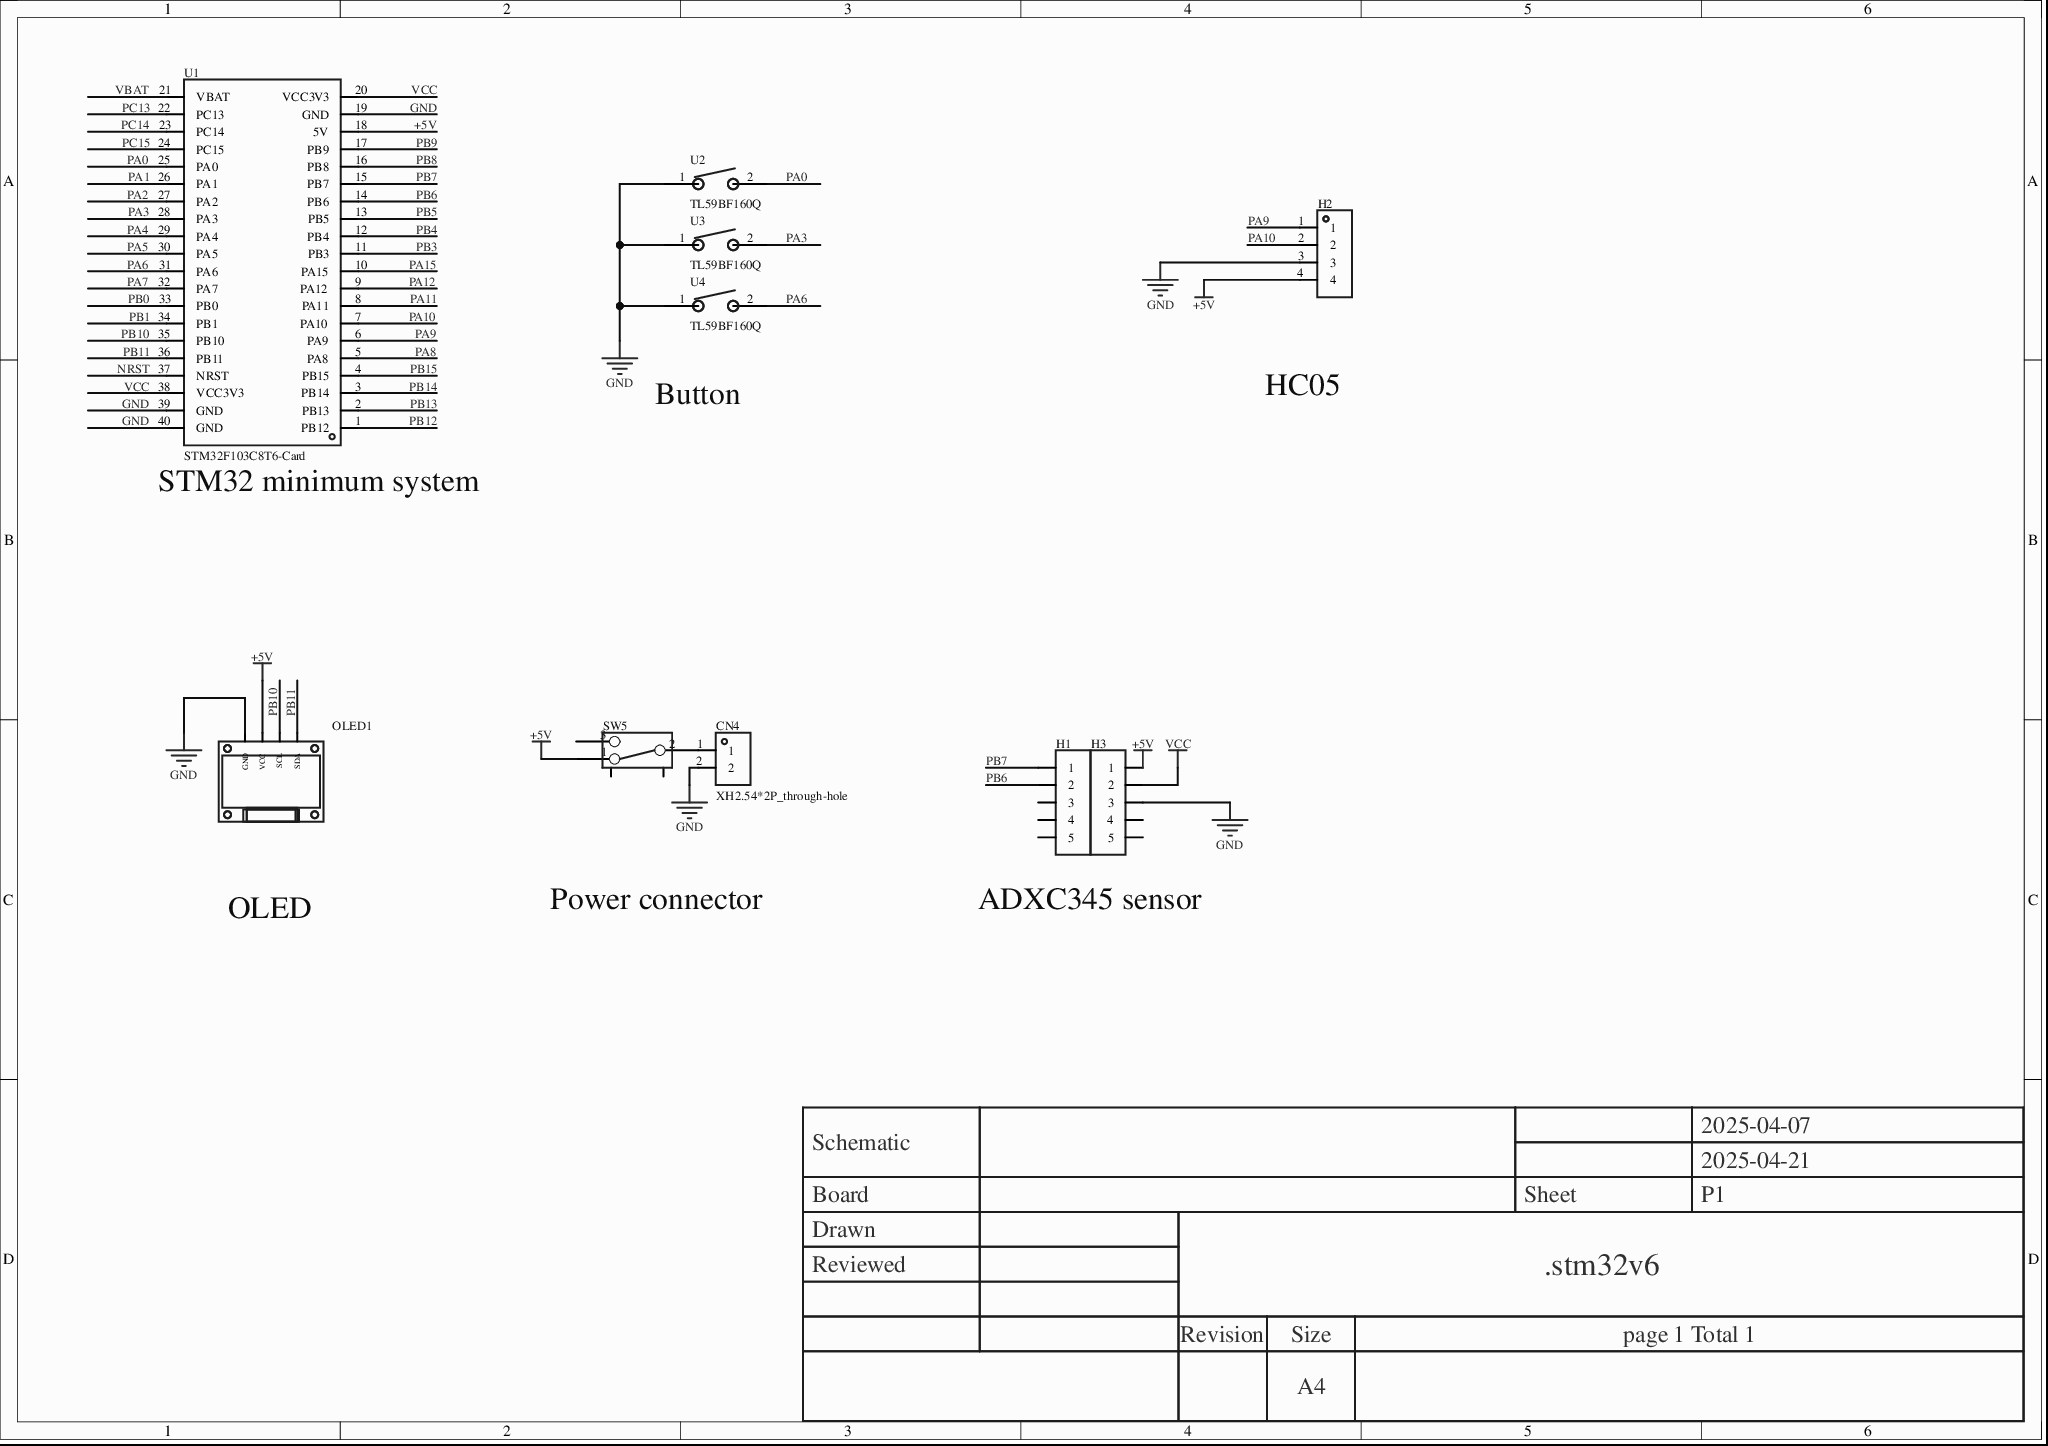
[diagram p0: MISC51878-3.schdoc]
# Altium project MISC51878-2.PrjPcb
1 sheet, 10 parts. Net scope: global (net labels, ports and power ports of the same name join across sheets).
Board file: MISC51878.pcbdoc

## Sheet MISC51878-3.schdoc
size 297 x 209 mm; Version: V1.0; @Project Name: MISC51878; @Page Count: 1; @Update Date: 2026-04-14; @Create Date: 2026-04-14; @Schematic Name: MISC51878; @Page No: 1; @Create Time: 23:22:16; @Update Time: 17:32:40; @Board Name: MISC51878

### Parts
CN4  XH2.54*2P_through-hole  [CONN-TH_2P-P2.50-XH2.54-2P]
H1  (no value)  [HDR-TH_5P-P2.54-V-F]
H2  (no value)  [HDR-TH_4P-P2.54-V-F]
H3  (no value)  [HDR-TH_5P-P2.54-V-F]
OLED1  (no value)  [0.96OLED_4P]
SW5  (no value)  [拨动开关]
U1  STM32F103C8T6-Card  [CONN-TH_L53.3-W22.9_STM32F103C8T6-CARD]
U2  TL59BF160Q  [KEY-TH_L6.2-W6.2-P5.00]
U3  TL59BF160Q  [KEY-TH_L6.2-W6.2-P5.00]
U4  TL59BF160Q  [KEY-TH_L6.2-W6.2-P5.00]

### Nets
+5V: H2.4 H3.1 OLED1.2(VCC) SW5.1 U1.18(5V)
GND: CN4.2 H2.3 H3.3 OLED1.1(GND) U1.19(GND) U1.39(GND) U1.40(GND) U2.1 U3.1 U4.1
VCC: H3.2 U1.20(VCC3V3) U1.38(VCC3V3)
NRST: U1.37(NRST)
PA0: U1.25(PA0) U2.2
PA1: U1.26(PA1)
PA2: U1.27(PA2)
PA3: U1.28(PA3) U3.2
PA4: U1.29(PA4)
PA5: U1.30(PA5)
PA6: U1.31(PA6) U4.2
PA7: U1.32(PA7)
PA8: U1.5(PA8)
PA9: H2.1 U1.6(PA9)
PA10: H2.2 U1.7(PA10)
PA11: U1.8(PA11)
PA12: U1.9(PA12)
PA15: U1.10(PA15)
PB0: U1.33(PB0)
PB1: U1.34(PB1)
PB3: U1.11(PB3)
PB4: U1.12(PB4)
PB5: U1.13(PB5)
PB6: H1.2 U1.14(PB6)
PB7: H1.1 U1.15(PB7)
PB8: U1.16(PB8)
PB9: U1.17(PB9)
PB10: OLED1.3(SCL) U1.35(PB10)
PB11: OLED1.4(SDA) U1.36(PB11)
PB12: U1.1(PB12)
PB13: U1.2(PB13)
PB14: U1.3(PB14)
PB15: U1.4(PB15)
PC13: U1.22(PC13)
PC14: U1.23(PC14)
PC15: U1.24(PC15)
VBAT: U1.21(VBAT)
NetCN4_1: CN4.1 SW5.2

Not connected (* = marked no-connect by the designer): H1 3 4 5; H3 4 5; SW5 3 4 5

### Notes on the sheet
- Button
- HC05
- (near U1) STM32 minimum system
- OLED
- Power connector
- ADXC345 sensor
- 2025-04-07
- Schematic
- Board
- Sheet
- 2025-04-21
- P1
- Drawn
- Reviewed
- .stm32v6
- Revision
- Size
- A4
- page 1 Total 1

### Library data of the parts
CN4 = XH2.54*2P_直插: 3D Model: 325c595e30db4df8abe76612dd40b0fa0819f05c4eef4c71ace90d822a990e87; 3D Model Transform: 295.275,228.346,0,180,0,0,-0.002,-20.079,-137.795; AddInBom: yes; Device: XH2.54*2P_through-hole; Symbol: XH2.54*2P_through-hole; LCSC Part Name: XH2.54*2P_直插; Supplier Part: C9900008615; Manufacturer Part: XH2.54*2P_直插; Supplier Footprint: XH2.54_2P; JLCPCB Part Class: Extended Part; Supplier: LCSC; FootprintName: CONN-TH_2P-P2.50-XH2.54-2P; ConvertToPcb: yes; ModelName: CONN-TH_2P-P2.50-XH2.54-2P
H1 H3 = HDR-F_2.54_1x5P: Symbol: Header-Female-2.54_1x5; ConvertToPcb: yes; ModelId: f49cb6116a3d45e5a64915bf3e00773f; ModelTransform: 519.684,98.464,0,0,0,0,0,0,-124.016; Device: HDR-F_2.54_1x5P; AddInBom: yes; SupplierPart: C50950; Supplier Footprint: 插件; FootprintName: HDR-TH_5P-P2.54-V-F; ModelName: HDR-TH_5P-P2.54-V-F
H2 = HDR-F_2.54_1x4P: Symbol: 2.54-1*4P female; ConvertToPcb: yes; ModelId: d187812051054f85879fcaa51a310d8e0819f05c4eef4c71ace90d822a990e87; ModelTransform: 419.6842,98.464,0,0,0,0,0,0,-118.11; Device: HDR-F_2.54_1x4P; FootprintName: HDR-TH_4P-P2.54-V-F; AddInBom: yes; SupplierPart: C2718488; Supplier Footprint: 插件; ModelName: HDR-TH_4P-P2.54-V-F
OLED1 = 0.96OLED模块_4P: Device: 0.96OLED module_4P; ConvertToPcb: yes; ModelId: 79c000fdb68d45a296c2e9bedf4f9055; ModelTransform: 1393.69792,1318.895,0,0,0,0,0,-560.079,-137.795; Symbol: 0.96OLED module_4P; FootprintName: 0.96OLED_4P; AddInBom: yes; Supplier Footprint: 插件; ModelName: 0.96OLED_4P
SW5 = 拨动开关_正: Device: Toggle switch_positive; Symbol: Toggle switch; ConvertToPcb: yes; ModelId: 4321fe59a4074cbfb4989553f297c68f0819f05c4eef4c71ace90d822a990e87; ModelName: SW-TH_SS-12D02-VG4; ModelTransform: 370.09,208.7,472.35,0,0,0,0,0,-110; FootprintName: Toggle switch; AddInBom: yes; Supplier Footprint: 插件
U1 = STM32F103C8T6-Card: AddInBom: yes; Device: STM32F103C8T6-Card; Symbol: STM32F103C8T6-CARD; FootprintName: CONN-TH_L53.3-W22.9_STM32F103C8T6-CARD; LCSC Part Name: STM32F103C8T6-Card; SupplierPart: C9900077949; ManufacturerPart: STM32F103C8T6-Card; Supplier Footprint: 插件; Supplier: LCSC; ConvertToPcb: yes
U2-U4 = TL59BF160Q: Circuit structure: SPST; button shape: round button; actuating force: 1.6N; mounting: through-hole; contact current: 50mA; rated voltage: 12V; service life: 10万 cycles;; Manufacturer: E-Switch; AddInBom: yes; ModelId: 1cf29b5a668b4918b807a6115220cae20819f05c4eef4c71ace90d822a990e87; ModelName: KEY-TH_L6.2-W6.2-H5.0-P5.0; ModelTransform: 244.094,244.094,0,0,0,0,0,0,-137.795; Symbol: TL59BF160Q; Device: TL59BF160Q; LCSC Part Name: TL59BF160Q; SupplierPart: C4364280; ManufacturerPart: TL59BF160Q; Supplier Footprint: 插件; JLCPCB Part Class: Extended Part; Datasheet: https://atta.szlcsc.com/upload/public/pdf/source/20231023/TL59-TL58.pdf-10f214b9358edf7c1c09f7d3f64515fe.pdf; Supplier: LCSC; ConvertToPcb: yes; FootprintName: KEY-TH_L6.2-W6.2-P5.00; Circuit: SPST; Actuator Style: Round button; Operating Force: 1.6N; Mounting Type: Through-hole; Contact Current: 50mA; Voltage Rating: 12V; IP Rating: -; Termination Style: PC pin; Life: 10万 cycles; Operating Temperature: -20℃~+70℃